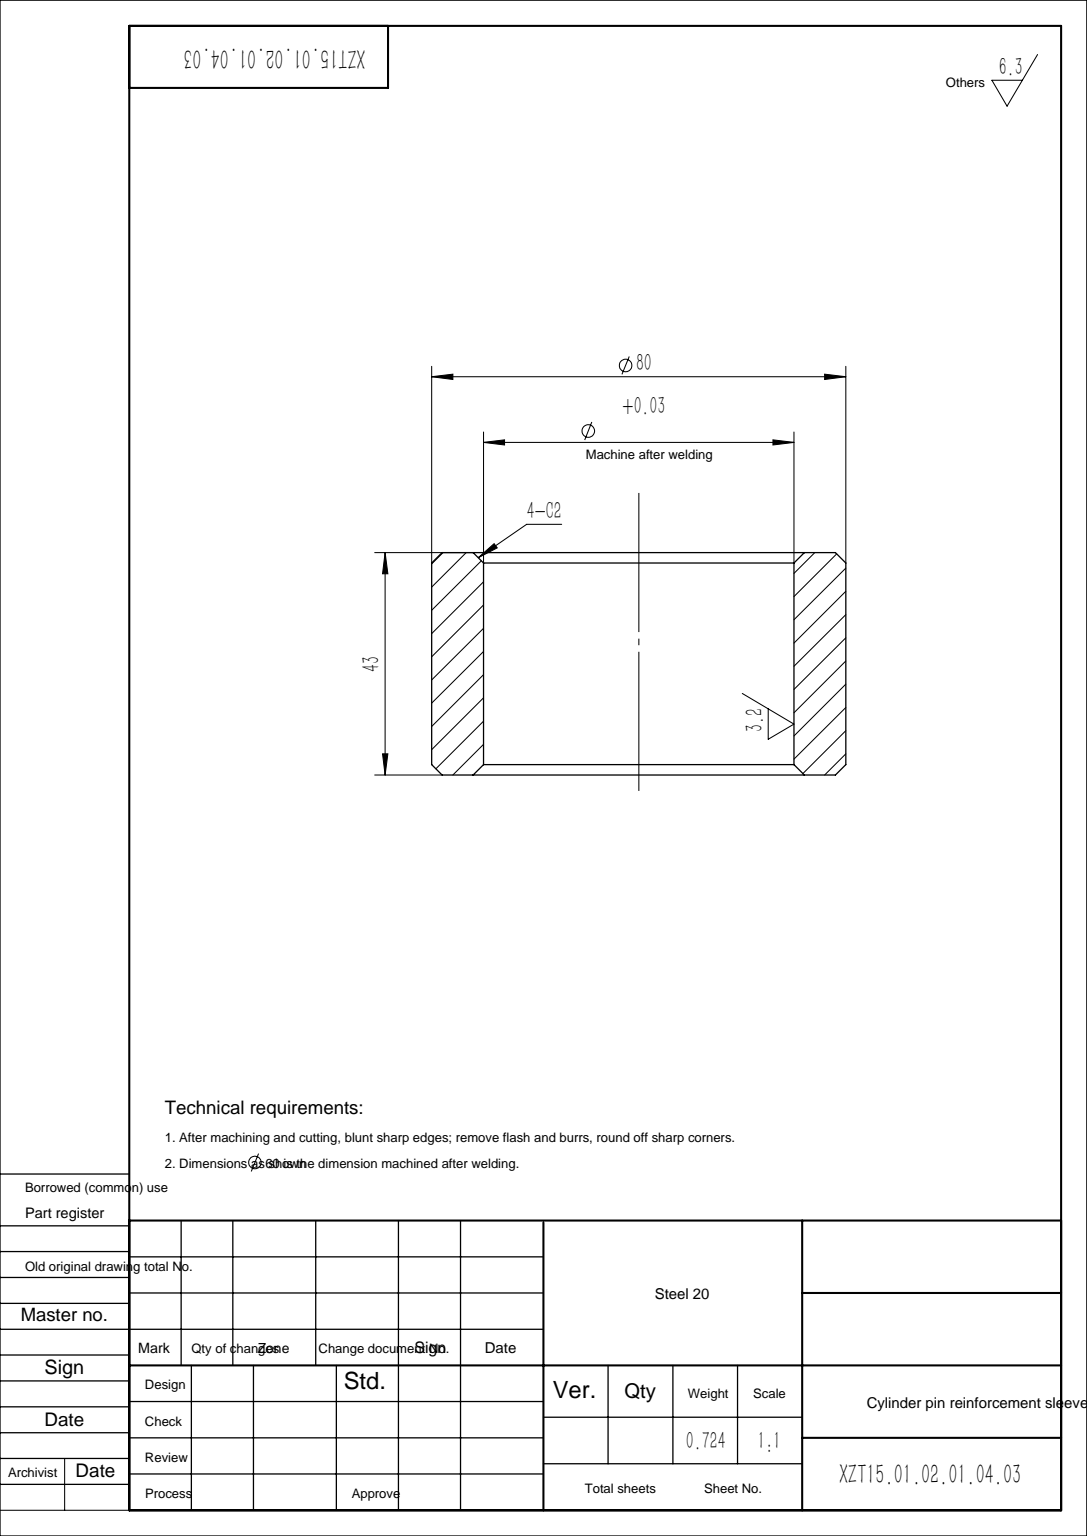
SolidWorks part; units mm, degrees
material "20 Steel"
ref_plane "Front Plane" through (0, 0, 0) normal (0, 0, 1) x (1, 0, 0)
ref_plane "Top Plane" through (0, 0, 0) normal (0, 1, 0) x (1, 0, 0)
ref_plane "Right Plane" through (0, 0, 0) normal (1, 0, 0) x (0, 0, -1)
sketch "Sketch1" plane through (0, 0, 0) normal (0, 1, 0) x (1, 0, 0)
  circle A0 centre (0, 0) radius 30
  circle A1 centre (0, 0) radius 40
  dimension "D1" = 60
  dimension "D2" = 80
extrude "Boss-Extrude1" add sketch "Sketch1" along normal blind 43
chamfer "Chamfer2" distance 2 angle 45 4 edges at (0, 0, 30) (0, 43, 30) (0, 0, 40) (0, 43, 40)
